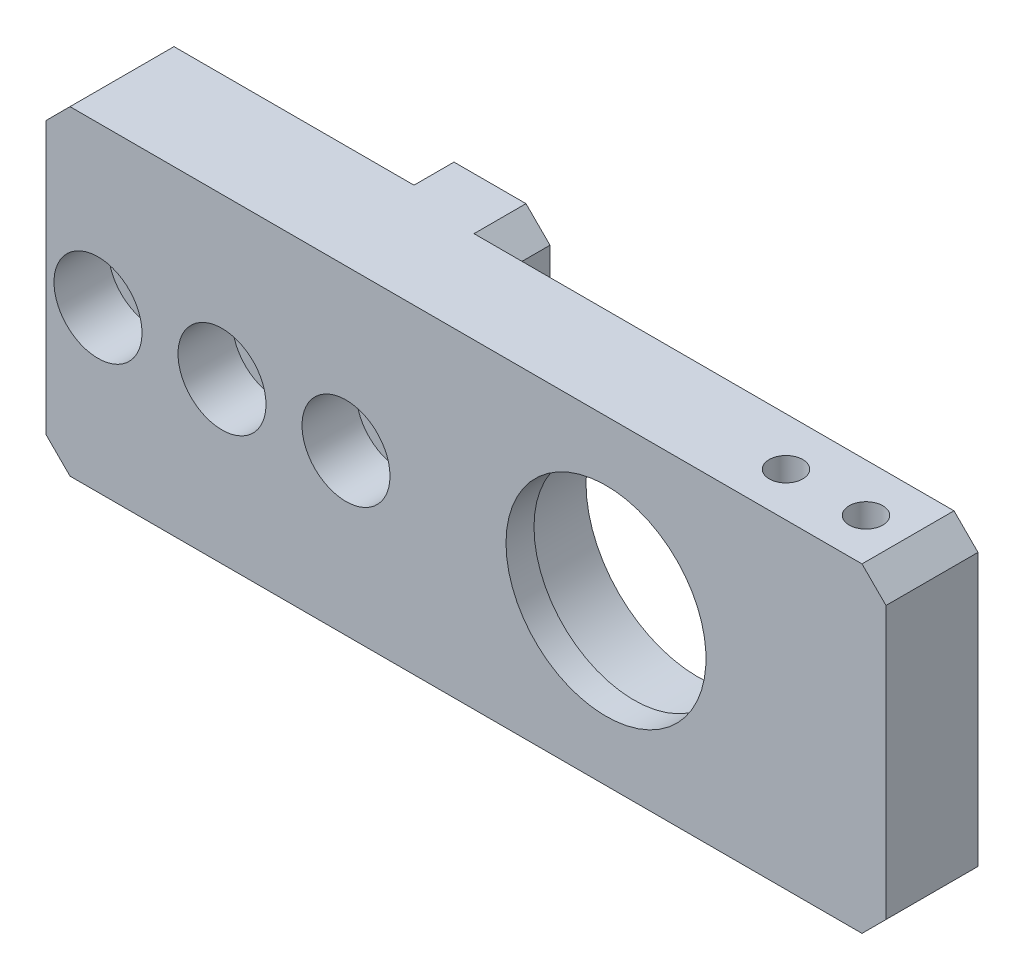
from build123d import *

# Parameters (mm, degrees)
SKETCH_1_W                  = 105
SKETCH_1_H                  = 40
EXTRUDE_1_DEPTH             = 18
SKETCH_2_W                  = 30
SKETCH_2_H                  = 40
CUT_EXTRUDE_1_DEPTH         = 5
SKETCH_3_W                  = 60
SKETCH_3_H                  = 40
CUT_EXTRUDE_2_DEPTH         = 6.5
HOLE_WIZARD_1_D             = 6.6
HOLE_WIZARD_1_CBORE_D       = 11
HOLE_WIZARD_1_CBORE_DEPTH   = 6.8
SKETCH_6_R                  = 5
CUT_EXTRUDE_3_DEPTH         = 2
SKETCH_7_R                  = 14
CUT_EXTRUDE_4_DEPTH         = 8
SKETCH_8_R                  = 12.5
CUT_EXTRUDE_5_DEPTH         = 59.021547722
CHAMFER_1_SIZE              = 3
HOLE_WIZARD_M5_1_AT_2_COUNT = 2
HOLE_WIZARD_M5_1_AT_2_PITCH = 10


with BuildPart() as part:
    # 草图1 → 凸台-拉伸1 (new body)
    with BuildSketch(Plane.XY):
        Rectangle(SKETCH_1_W, SKETCH_1_H)
    extrude(amount=EXTRUDE_1_DEPTH)

    # 草图2 → 切除-拉伸1 (cut)
    with BuildSketch(Plane(origin=(0, 0, 0), x_dir=(-1, 0, 0), z_dir=(0, 0, -1))):
        with Locations((37.5, 0)):
            Rectangle(SKETCH_2_W, SKETCH_2_H)
    extrude(amount=-CUT_EXTRUDE_1_DEPTH, mode=Mode.SUBTRACT)

    # 草图3 → 切除-拉伸2 (cut)
    with BuildSketch(Plane(origin=(0, 0, 0), x_dir=(-1, 0, 0), z_dir=(0, 0, -1))):
        with Locations((-22.5, 0)):
            Rectangle(SKETCH_3_W, SKETCH_3_H)
    extrude(amount=-CUT_EXTRUDE_2_DEPTH, mode=Mode.SUBTRACT)

    # 打孔尺寸(%根据)内六角圆柱头螺钉的类型1 (through all)
    with Locations(Plane.XY.offset(18)):
        with Locations((-46, 0), (-30.5, 0), (-15, 0)):
            CounterBoreHole(HOLE_WIZARD_1_D / 2, HOLE_WIZARD_1_CBORE_D / 2, HOLE_WIZARD_1_CBORE_DEPTH)

    # 草图6 → 切除-拉伸3 (cut)
    with BuildSketch(Plane(origin=(0, 0, 0), x_dir=(-1, 0, 0), z_dir=(0, 0, -1))):
        with Locations((15, 0)):
            Circle(SKETCH_6_R)
    extrude(amount=-CUT_EXTRUDE_3_DEPTH, mode=Mode.SUBTRACT)

    # 草图7 → 切除-拉伸4 (cut)
    with BuildSketch(Plane(origin=(0, 0, 6.5), x_dir=(-1, 0, 0), z_dir=(0, 0, -1))):
        with Locations((-17.5, 0)):
            Circle(SKETCH_7_R)
    extrude(amount=-CUT_EXTRUDE_4_DEPTH, mode=Mode.SUBTRACT)

    # 草图8 → 切除-拉伸5 (cut, through all)
    with BuildSketch(Plane(origin=(0, 0, 14.5), x_dir=(-1, 0, 0), z_dir=(0, 0, -1))):
        with Locations((-17.5, 0)):
            Circle(SKETCH_8_R)
    extrude(amount=-CUT_EXTRUDE_5_DEPTH, mode=Mode.SUBTRACT)

    # 倒角1
    chamfer_1_edges = [part.edges().sort_by_distance(p)[0] for p in [
        (-22.5, -20, 2.5),
        (-22.5, 20, 2.5),
        (-7.5, 20, 3.25),
        (-7.5, -20, 3.25),
        (52.5, -20, 12.25),
        (-52.5, -20, 11.5),
        (-52.5, 20, 11.5),
        (52.5, 20, 12.25),
    ]]
    chamfer(chamfer_1_edges, length=CHAMFER_1_SIZE)

    # 草图10 → M5 螺纹孔1 (revolve, cut)
    with BuildSketch(Plane(origin=(44.5, -20, 12.5), x_dir=(0, 0, -1), z_dir=(1, 0, 0))):
        Polygon((0, 0), (0, 13.6618073), (2.1, 12.4), (2.1, 0), align=None)
    hole_wizard_m5_1 = revolve(axis=Axis((44.5, -26.35, 12.5), (0, 1, 0)), mode=Mode.SUBTRACT)

    # M5 螺纹孔1 at 2: M5 螺纹孔1 ×2
    with Locations(*[(-i * HOLE_WIZARD_M5_1_AT_2_PITCH, 0, 0) for i in range(1, HOLE_WIZARD_M5_1_AT_2_COUNT)]):
        add(hole_wizard_m5_1, mode=Mode.SUBTRACT)

    # 镜向1: M5 螺纹孔1 across plane
    add(hole_wizard_m5_1.mirror(Plane.ZX), mode=Mode.SUBTRACT)

    # 镜向1 copy 1 sketch → 镜向1 copy 1 (revolve, cut)
    with BuildSketch(Plane(origin=(34.5, 20, 12.5), x_dir=(0, 0, -1), z_dir=(1, 0, 0))):
        Polygon((0, 0), (0, -13.6618073), (2.1, -12.4), (2.1, 0), align=None)
    revolve(axis=Axis((34.5, 26.35, 12.5), (0, 1, 0)), mode=Mode.SUBTRACT)


solid = part.part
